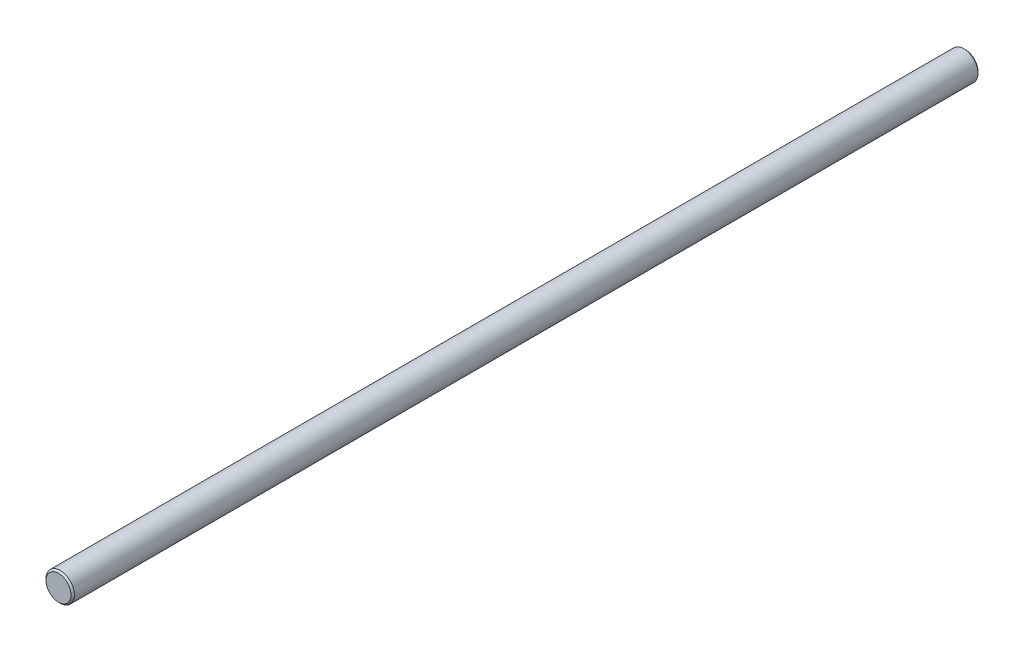
from build123d import *

# Parameters (mm, degrees)
SKETCH1_R           = 4.25
BOSS_EXTRUDE1_DEPTH = 271.5
CHAMFER1_SIZE       = 0.5


with BuildPart() as part:
    # Sketch1 → Boss-Extrude1 (new body)
    with BuildSketch(Plane.XY):
        Circle(SKETCH1_R)
    extrude(amount=BOSS_EXTRUDE1_DEPTH)

    # Chamfer1
    chamfer1_edges = [part.edges().sort_by_distance(p)[0] for p in [
        (-4.25, 0, 0),
        (-4.25, 0, 271.5),
    ]]
    chamfer(chamfer1_edges, length=CHAMFER1_SIZE)


solid = part.part
